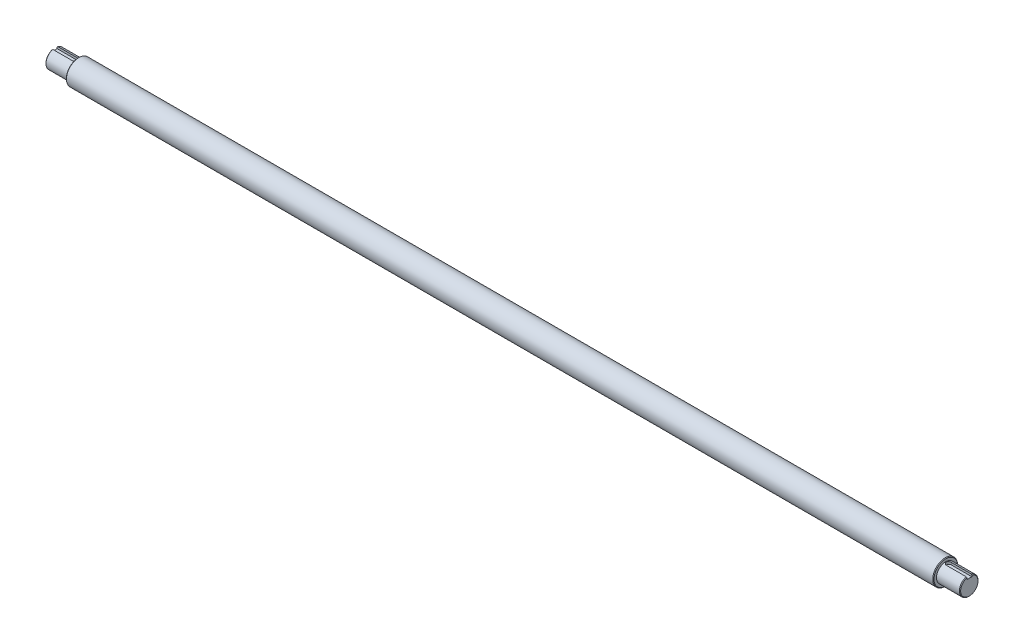
from build123d import *

# Parameters (mm, degrees)
CUT_EXTRUDE1_DEPTH = 4
CHAMFER1_SIZE      = 1


with BuildPart() as part:
    # Sketch1 → Revolve1 (revolve)
    with BuildSketch(Plane.XY, mode=Mode.PRIVATE) as revolve1_sk:
        Polygon((-738, 15), (-700, 15), (-700, 20), (700, 20), (700, 15), (738, 15), (738, 0), (-738, 0), align=None)
    revolve(revolve1_sk.sketch.rotate(Axis((738, 0, 0), (-1, 0, 0)), 90), axis=Axis((738, 0, 0), (-1, 0, 0)))

    # Sketch3 → Cut-Extrude1 (cut)
    with BuildSketch(Plane(origin=(0, 15, 0), x_dir=(1, 0, 0), z_dir=(0, 1, 0))):
        with BuildLine():
            Line((-705, 4), (-738, 4))
            Line((-738, 4), (-738, -4))
            Line((-738, -4), (-705, -4))
            ThreePointArc((-705, -4), (-701, 0), (-705, 4))
        make_face()
    cut_extrude1 = extrude(amount=-CUT_EXTRUDE1_DEPTH, mode=Mode.SUBTRACT)

    # Mirror1: Cut-Extrude1 across plane
    add(cut_extrude1.mirror(Plane.ZY), mode=Mode.SUBTRACT)

    # Chamfer1
    chamfer1_edges = [part.edges().sort_by_distance(p)[0] for p in [
        (-738, -11.937336386, 9.082951062),
        (738, -11.937336386, 9.082951062),
        (700, 0, 20),
        (-700, 0, 20),
    ]]
    chamfer(chamfer1_edges, length=CHAMFER1_SIZE)


solid = part.part
